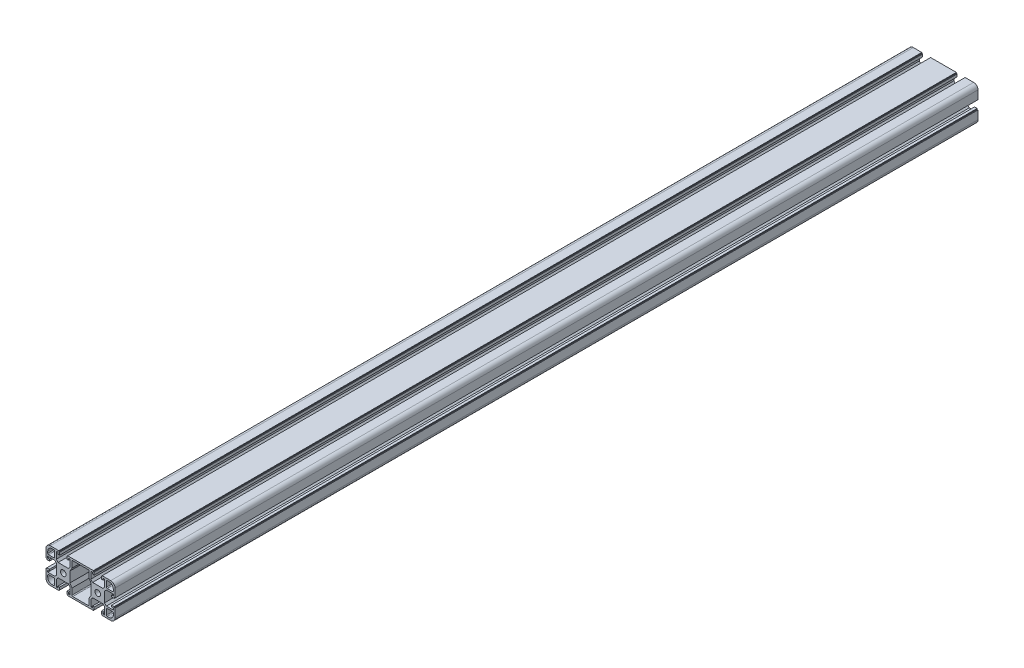
from build123d import *

# Parameters (mm, degrees)
SKETCH_1_R      = 3.25
SKETCH_1_W      = 8
SKETCH_1_H      = 8
EXTRUDE_1_DEPTH = 1000
FILLET_1_R      = 5
FILLET_2_R      = 1


with BuildPart() as part:
    # 草图1 → 拉伸1 (new body)
    with BuildSketch(Plane.XY):
        Polygon((-5.1, 20), (-5.1, 19), (-4.1, 19), (-4.1, 16), (-6.1, 16), (-6.1, 18), (-8, 18), (-8, 10), (-6, 7.7), (6, 7.7), (8, 10), (8, 18), (6.1, 18), (6.1, 16), (4.1, 16), (4.1, 19), (5.1, 19), (5.1, 20), (34.9, 20), (34.9, 19), (35.9, 19), (35.9, 16), (33.9, 16), (33.9, 18), (32, 18), (32, 10), (34, 7.7), (46, 7.7), (48, 10), (48, 18), (46.1, 18), (46.1, 16), (44.1, 16), (44.1, 19), (45.1, 19), (45.1, 20), (60, 20), (60, 5.1), (59, 5.1), (59, 4.1), (56, 4.1), (56, 6.1), (58, 6.1), (58, 8), (50, 8), (47.7, 6), (47.7, -6), (50, -8), (58, -8), (58, -6.1), (56, -6.1), (56, -4.1), (59, -4.1), (59, -5.1), (60, -5.1), (60, -20), (45.1, -20), (45.1, -19), (44.1, -19), (44.1, -16), (46.1, -16), (46.1, -18), (48, -18), (48, -10), (46, -7.7), (34, -7.7), (32, -10), (32, -18), (33.9, -18), (33.9, -16), (35.9, -16), (35.9, -19), (34.9, -19), (34.9, -20), (5.1, -20), (5.1, -19), (4.1, -19), (4.1, -16), (6.1, -16), (6.1, -18), (8, -18), (8, -10), (6, -7.7), (-6, -7.7), (-8, -10), (-8, -18), (-6.1, -18), (-6.1, -16), (-4.1, -16), (-4.1, -19), (-5.1, -19), (-5.1, -20), (-20, -20), (-20, -5.1), (-19, -5.1), (-19, -4.1), (-16, -4.1), (-16, -6.1), (-18, -6.1), (-18, -8), (-10, -8), (-7.7, -6), (-7.7, 6), (-10, 8), (-18, 8), (-18, 6.1), (-16, 6.1), (-16, 4.1), (-19, 4.1), (-19, 5.1), (-20, 5.1), (-20, 20), align=None)
        Circle(SKETCH_1_R, mode=Mode.SUBTRACT)
        with Locations(Location((40, 0, 0), (0, 0, 180))):
            Circle(SKETCH_1_R, mode=Mode.SUBTRACT)
        Polygon((7.7, 6), (10, 10), (10, 18), (30, 18), (30, 10), (32.3, 6), (32.3, -6), (30, -10), (30, -18), (10, -18), (10, -10), (7.7, -6), align=None, mode=Mode.SUBTRACT)
        with Locations((-14, 14)):
            Rectangle(SKETCH_1_W, SKETCH_1_H, mode=Mode.SUBTRACT)
        with Locations((-14, -14)):
            Rectangle(SKETCH_1_W, SKETCH_1_H, mode=Mode.SUBTRACT)
        with Locations((54, -14)):
            Rectangle(SKETCH_1_W, SKETCH_1_H, mode=Mode.SUBTRACT)
        with Locations((54, 14)):
            Rectangle(SKETCH_1_W, SKETCH_1_H, mode=Mode.SUBTRACT)
    extrude(amount=EXTRUDE_1_DEPTH)

    # 圆角1
    fillet_1_edges = [part.edges().sort_by_distance(p)[0] for p in [
        (-20, 20, 500),
        (60, 20, 500),
        (60, -20, 500),
        (-20, -20, 500),
        (-18, 18, 500),
        (-18, -18, 500),
        (58, -18, 500),
        (58, 18, 500),
    ]]
    fillet(fillet_1_edges, radius=FILLET_1_R)

    # 圆角2
    fillet_2_edges = [part.edges().sort_by_distance(p)[0] for p in [
        (10, -18, 500),
        (30, -18, 500),
        (30, 18, 500),
        (10, 18, 500),
        (-18, 10, 500),
        (-10, 10, 500),
        (-10, 18, 500),
        (-10, -18, 500),
        (-10, -10, 500),
        (-18, -10, 500),
        (58, -10, 500),
        (50, -10, 500),
        (50, -18, 500),
        (50, 18, 500),
        (50, 10, 500),
        (58, 10, 500),
    ]]
    fillet(fillet_2_edges, radius=FILLET_2_R)


solid = part.part
